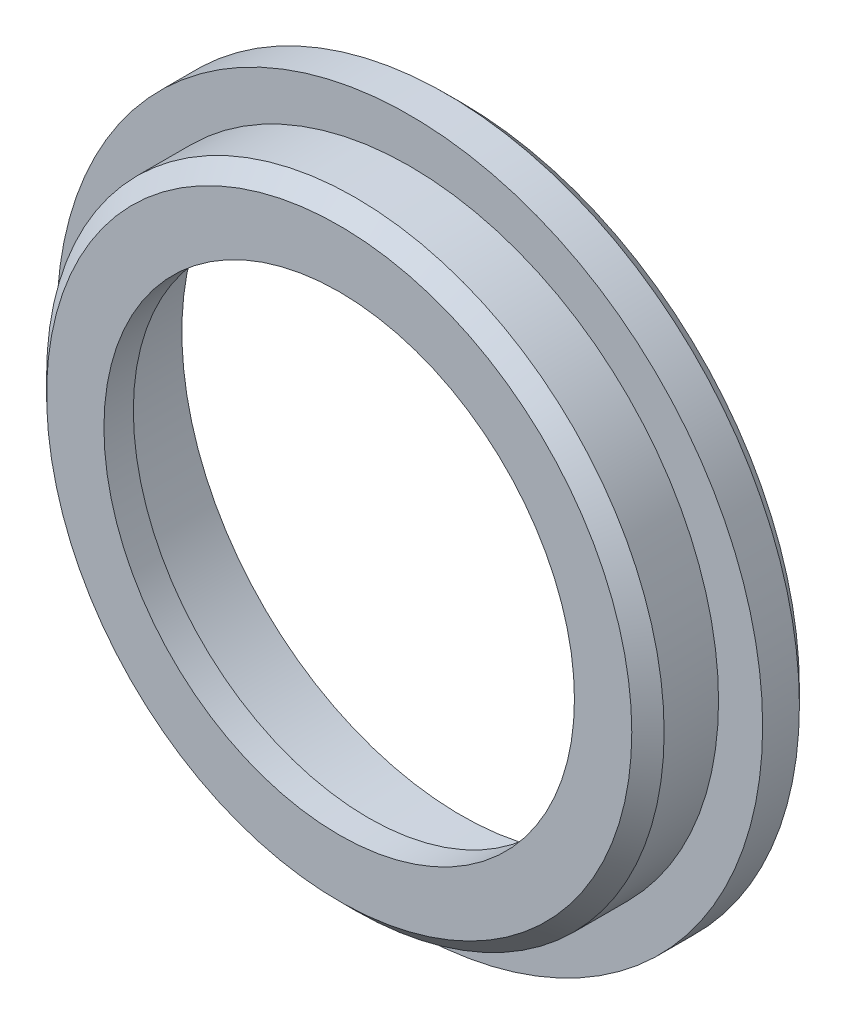
from build123d import *

# Parameters (mm, degrees)
SKETCH_1_R      = 24
SKETCH_1_R_2    = 19
EXTRUDE_1_DEPTH = 3.5
SKETCH_2_R      = 21
SKETCH_2_R_2    = 19
EXTRUDE_2_DEPTH = 2.8
SKETCH_3_R      = 21
SKETCH_3_R_2    = 16
EXTRUDE_3_DEPTH = 2
CHAMFER_1_SIZE  = 1.1
CHAMFER_2_SIZE  = 1


with BuildPart() as part:
    # 草图1 → 凸台-拉伸1 (new body)
    with BuildSketch(Plane.XY):
        Circle(SKETCH_1_R)
        Circle(SKETCH_1_R_2, mode=Mode.SUBTRACT)
    extrude(amount=EXTRUDE_1_DEPTH)

    # 草图2 → 凸台-拉伸2 (add)
    with BuildSketch(Plane.XY.offset(3.5)):
        Circle(SKETCH_2_R)
        Circle(SKETCH_2_R_2, mode=Mode.SUBTRACT)
    extrude(amount=EXTRUDE_2_DEPTH)

    # 草图3 → 凸台-拉伸3 (add)
    with BuildSketch(Plane.XY.offset(6.3)):
        Circle(SKETCH_3_R)
        Circle(SKETCH_3_R_2, mode=Mode.SUBTRACT)
    extrude(amount=EXTRUDE_3_DEPTH)

    # 倒角1
    chamfer_1_edges = [part.edges().sort_by_distance(p)[0] for p in [
        (-21, 0, 8.3),
        (-19, 0, 6.3),
    ]]
    chamfer(chamfer_1_edges, length=CHAMFER_1_SIZE)

    # 倒角2
    chamfer_2_edges = [part.edges().sort_by_distance(p)[0] for p in [
        (-24, 0, 0),
    ]]
    chamfer(chamfer_2_edges, length=CHAMFER_2_SIZE)


solid = part.part
